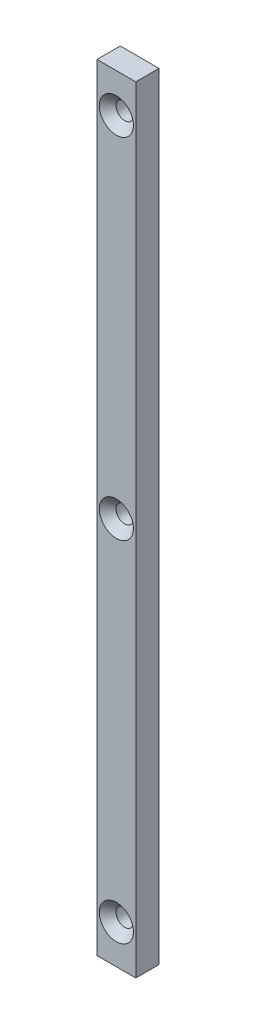
from build123d import *

# Parameters (mm, degrees)
SKETCH1_W                                           = 20
SKETCH1_H                                           = 400
BOSS_EXTRUDE1_DEPTH                                 = 12
HOLE_SIZE_BY_HEX_SOCKET_FLAT_COUNTERSUN_D           = 9
HOLE_SIZE_BY_HEX_SOCKET_FLAT_COUNTERSUN_CSINK_D     = 17.6
HOLE_SIZE_BY_HEX_SOCKET_FLAT_COUNTERSUN_CSINK_ANGLE = 90


with BuildPart() as part:
    # Sketch1 → Boss-Extrude1 (new body)
    with BuildSketch(Plane.XY):
        with Locations((10, 200)):
            Rectangle(SKETCH1_W, SKETCH1_H)
    extrude(amount=BOSS_EXTRUDE1_DEPTH)

    # Hole size (by hex socket flat countersunk head screw type)1 (through all)
    with Locations(Plane.XY.offset(12)):
        with Locations((10, 380), (10, 200), (10, 20)):
            CounterSinkHole(HOLE_SIZE_BY_HEX_SOCKET_FLAT_COUNTERSUN_D / 2, HOLE_SIZE_BY_HEX_SOCKET_FLAT_COUNTERSUN_CSINK_D / 2, counter_sink_angle=HOLE_SIZE_BY_HEX_SOCKET_FLAT_COUNTERSUN_CSINK_ANGLE)


solid = part.part
